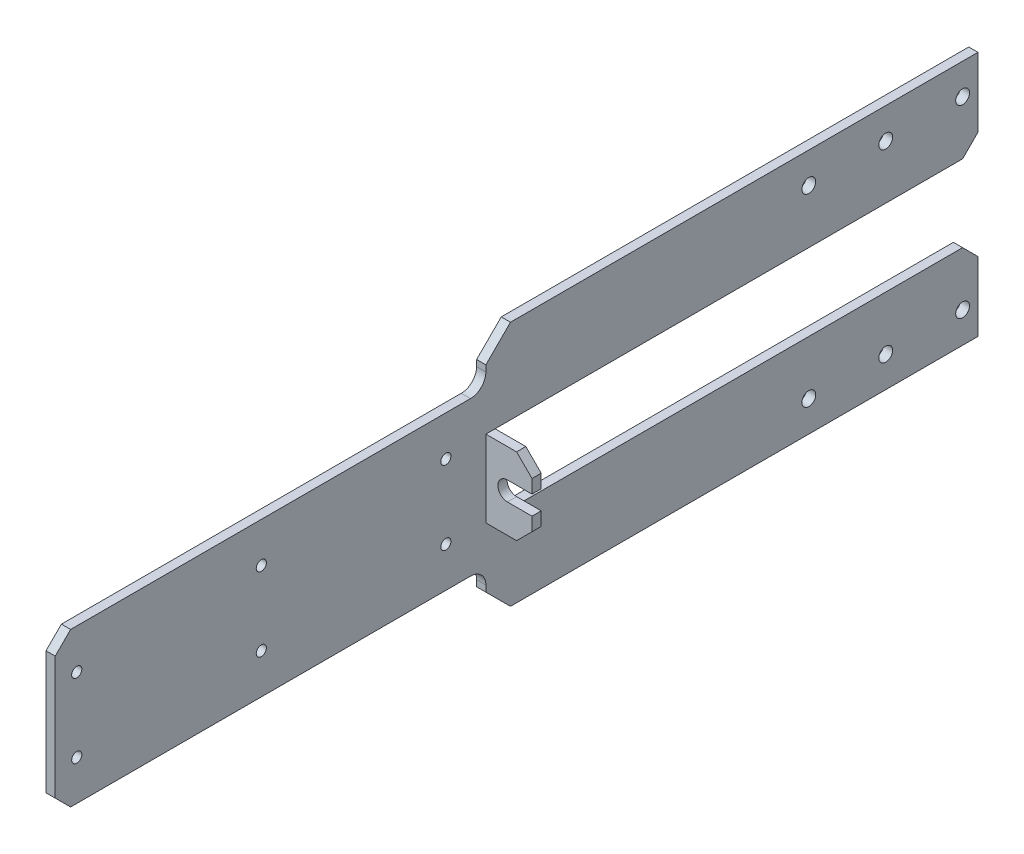
from build123d import *

# Parameters (mm, degrees)
BOSS_EXTRUDE1_DEPTH        = 80
SKETCH2_R                  = 2.75
CUT_EXTRUDE1_DEPTH         = 10
SKETCH3_W                  = 314
SKETCH3_H                  = 25
CUT_EXTRUDE2_DEPTH         = 10
SKETCH4_W                  = 140
SKETCH4_H                  = 50
BOSS_EXTRUDE2_DEPTH        = 3
SKETCH5_W                  = 24.712329927
SKETCH5_H                  = 27.5
CUT_EXTRUDE3_DEPTH         = 15
CHAMFER1_SIZE              = 5
CHAMFER2_SIZE              = 8
CUT_EXTRUDE4_DEPTH         = 112
SKETCH9_R                  = 1
CUT_EXTRUDE5_DEPTH         = 10
M4_TAPPED_HOLE1_AT_2_COUNT = 2
M4_TAPPED_HOLE1_AT_2_PITCH = 24
LPATTERN1_COUNT            = 3
LPATTERN1_PITCH            = 60
SKETCH11_R                 = 2.25
CUT_EXTRUDE6_DEPTH         = 10
LPATTERN2_COUNT            = 3
LPATTERN2_PITCH            = 25
CHAMFER3_SIZE              = 5
CHAMFER4_SIZE              = 5
FILLET1_R                  = 5


with BuildPart() as part:
    # Sketch1 → Boss-Extrude1 (new body)
    with BuildSketch(Plane(origin=(0, 0, 0), x_dir=(1, 0, 0), z_dir=(0, 1, 0))):
        Polygon((0, 0), (18, 0), (18, 3), (3, 3), (3, 160), (0, 160), align=None)
    extrude(amount=BOSS_EXTRUDE1_DEPTH)

    # Sketch2 → Cut-Extrude1 (cut)
    with BuildSketch(Plane.XY):
        with Locations((10, 40)):
            Circle(SKETCH2_R)
    extrude(amount=-CUT_EXTRUDE1_DEPTH, mode=Mode.SUBTRACT)

    # Sketch3 → Cut-Extrude2 (cut)
    with BuildSketch(Plane.ZY):
        with Locations((-160, 40)):
            Rectangle(SKETCH3_W, SKETCH3_H)
    extrude(amount=-CUT_EXTRUDE2_DEPTH, mode=Mode.SUBTRACT)

    # Sketch4 → Boss-Extrude2 (add)
    with BuildSketch(Plane.ZY):
        with Locations((70, 40)):
            Rectangle(SKETCH4_W, SKETCH4_H)
    extrude(amount=-BOSS_EXTRUDE2_DEPTH)

    # Sketch5 → Cut-Extrude3 (cut)
    with BuildSketch(Plane(origin=(18, 0, 0), x_dir=(0, 0, -1), z_dir=(1, 0, 0))):
        with Locations((-2.356164964, 13.75)):
            Rectangle(SKETCH5_W, SKETCH5_H)
        with Locations((-2.356164964, 66.25)):
            Rectangle(SKETCH5_W, SKETCH5_H)
    extrude(amount=-CUT_EXTRUDE3_DEPTH, mode=Mode.SUBTRACT)

    # Chamfer1
    chamfer1_edges = [part.edges().sort_by_distance(p)[0] for p in [
        (18, 27.5, -1.5),
        (18, 52.5, -1.5),
    ]]
    chamfer(chamfer1_edges, length=CHAMFER1_SIZE)

    # Chamfer2
    chamfer2_edges = [part.edges().sort_by_distance(p)[0] for p in [
        (1.5, 0, 0),
        (1.5, 80, 0),
    ]]
    chamfer(chamfer2_edges, length=CHAMFER2_SIZE)

    # Sketch8 → Cut-Extrude4 (cut)
    with BuildSketch(Plane(origin=(0, 0, -3), x_dir=(-1, 0, 0), z_dir=(0, 0, -1))):
        with BuildLine():
            Line((-26, 43.1), (-10, 43.1))
            ThreePointArc((-10, 43.1), (-6.9, 40), (-10, 36.9))
            Line((-10, 36.9), (-26, 36.9))
            ThreePointArc((-26, 36.9), (-29.1, 40), (-26, 43.1))
        make_face()
    extrude(amount=-CUT_EXTRUDE4_DEPTH, mode=Mode.SUBTRACT)

    # Sketch9 → Cut-Extrude5 (cut)
    with BuildSketch(Plane.ZY):
        with Locations((133, 52)):
            Circle(SKETCH9_R)
        with Locations((133, 28)):
            Circle(SKETCH9_R)
    extrude(amount=-CUT_EXTRUDE5_DEPTH, mode=Mode.SUBTRACT)

    # Sketch10 → M4 Tapped Hole1 (revolve, cut)
    with BuildSketch(Plane(origin=(0, 52, 133), x_dir=(0, 0, 1), z_dir=(0, 1, 0))):
        Polygon((0, 0), (0, 11.091420021), (1.65, 10.1), (1.65, 0), align=None)
    m4_tapped_hole1 = revolve(axis=Axis((-6.35, 52, 133), (1, 0, 0)), mode=Mode.SUBTRACT)

    # M4 Tapped Hole1 at 2: M4 Tapped Hole1 ×2
    with Locations(*[(0, -i * M4_TAPPED_HOLE1_AT_2_PITCH, 0) for i in range(1, M4_TAPPED_HOLE1_AT_2_COUNT)]):
        add(m4_tapped_hole1, mode=Mode.SUBTRACT)

    # LPattern1: M4 Tapped Hole1 ×3
    with Locations(*[(0, 0, -i * LPATTERN1_PITCH) for i in range(1, LPATTERN1_COUNT)]):
        add(m4_tapped_hole1, mode=Mode.SUBTRACT)

    # LPattern1 copy 1 sketch → LPattern1 copy 1 (revolve, cut)
    with BuildSketch(Plane(origin=(0, 28, 73), x_dir=(0, 0, 1), z_dir=(0, 1, 0))):
        Polygon((0, 0), (0, 11.091420021), (1.65, 10.1), (1.65, 0), align=None)
    revolve(axis=Axis((-6.35, 28, 73), (1, 0, 0)), mode=Mode.SUBTRACT)

    # LPattern1 copy 2 sketch → LPattern1 copy 2 (revolve, cut)
    with BuildSketch(Plane(origin=(0, 28, 13), x_dir=(0, 0, 1), z_dir=(0, 1, 0))):
        Polygon((0, 0), (0, 11.091420021), (1.65, 10.1), (1.65, 0), align=None)
    revolve(axis=Axis((-6.35, 28, 13), (1, 0, 0)), mode=Mode.SUBTRACT)

    # Sketch11 → Cut-Extrude6 (cut)
    with BuildSketch(Plane.ZY):
        with Locations((-155, 70)):
            Circle(SKETCH11_R)
        with Locations((-155, 10)):
            Circle(SKETCH11_R)
    cut_extrude6 = extrude(amount=-CUT_EXTRUDE6_DEPTH, mode=Mode.SUBTRACT)

    # LPattern2: Cut-Extrude6 ×3
    with Locations(*[(0, 0, i * LPATTERN2_PITCH) for i in range(1, LPATTERN2_COUNT)]):
        add(cut_extrude6, mode=Mode.SUBTRACT)

    # Chamfer3
    chamfer3_edges = [part.edges().sort_by_distance(p)[0] for p in [
        (1.5, 52.5, -160),
        (1.5, 27.5, -160),
    ]]
    chamfer(chamfer3_edges, length=CHAMFER3_SIZE)

    # Chamfer4
    chamfer4_edges = [part.edges().sort_by_distance(p)[0] for p in [
        (1.5, 15, 140),
        (1.5, 65, 140),
    ]]
    chamfer(chamfer4_edges, length=CHAMFER4_SIZE)

    # Fillet1
    fillet1_edges = [part.edges().sort_by_distance(p)[0] for p in [
        (1.5, 15, 0),
        (1.5, 65, 0),
    ]]
    fillet(fillet1_edges, radius=FILLET1_R)


solid = part.part
